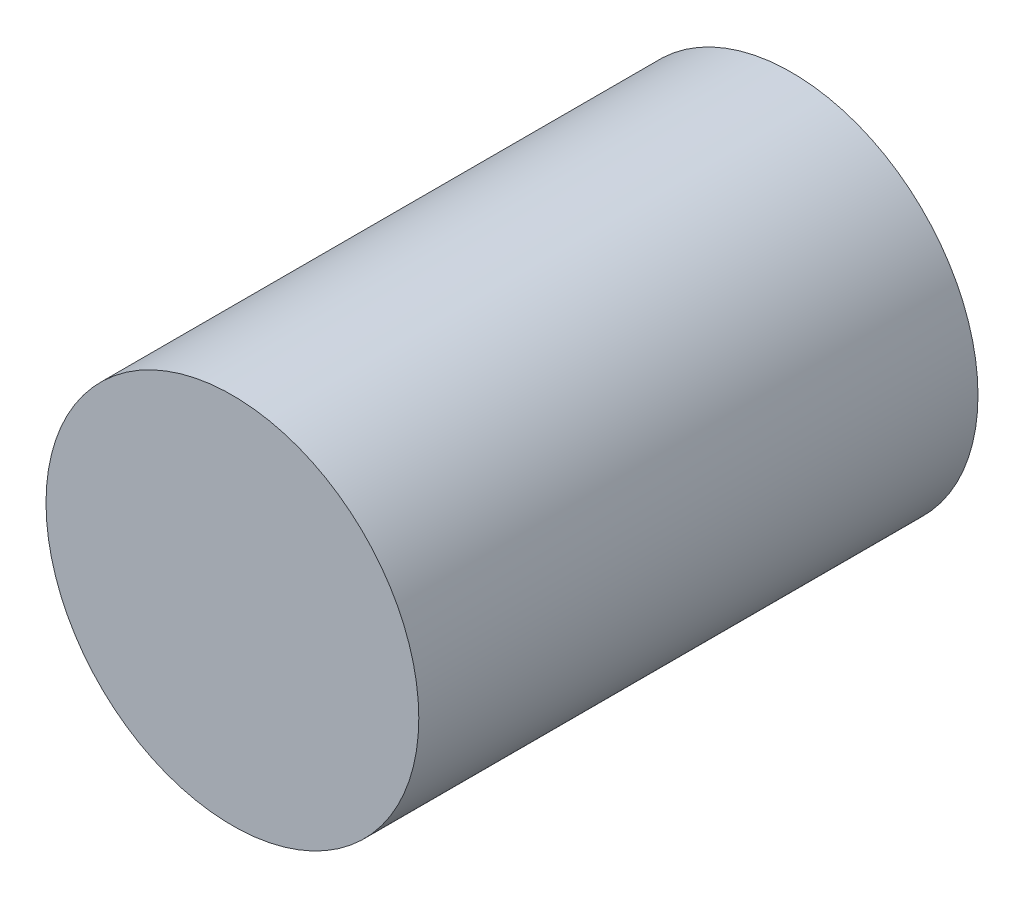
SolidWorks part; units mm, degrees
ref_plane "前视基准面" through (0, 0, 0) normal (0, 0, 1) x (1, 0, 0)
ref_plane "上视基准面" through (0, 0, 0) normal (0, 1, 0) x (1, 0, 0)
ref_plane "右视基准面" through (0, 0, 0) normal (1, 0, 0) x (0, 0, -1)
other "Configuration Table"
sketch "草图1" plane through (0, 0, 0) normal (0, 0, 1) x (1, 0, 0)
  circle A0 centre (0, 0) radius 4
  point P0 (0, 0)
  dimension "D1" = 8
extrude "凸台-拉伸1" add sketch "草图1" against normal mid plane 12
